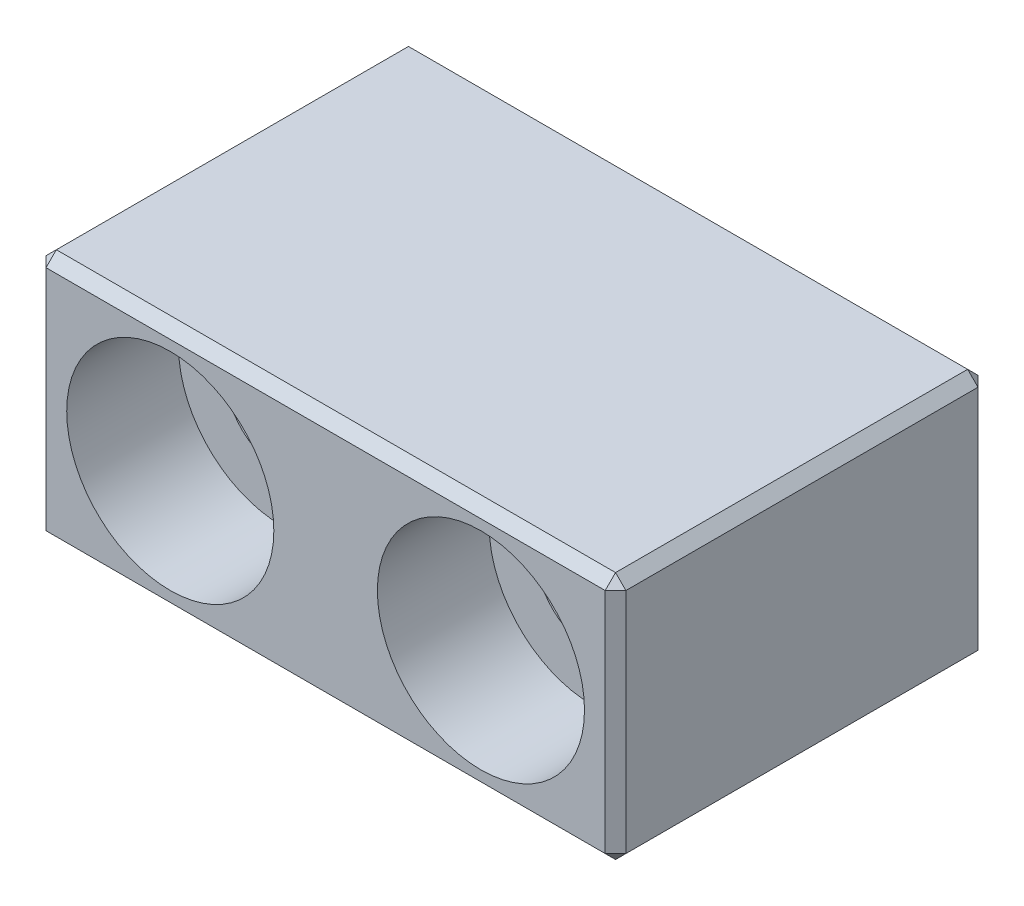
SolidWorks part; units mm, degrees
material "Al6061"
ref_plane "Front" through (0, 0, 0) normal (0, 0, 1) x (1, 0, 0)
ref_plane "Top" through (0, 0, 0) normal (0, 1, 0) x (1, 0, 0)
ref_plane "Right" through (0, 0, 0) normal (1, 0, 0) x (0, 0, -1)
sketch "草图1" plane through (0, 0, 0) normal (0, 1, 0) x (1, 0, 0)
  line L1 (-14, 9) -> (14, 9)
  line L2 (-14, 9) -> (-14, -9)
  line L3 (-14, -9) -> (14, -9)
  line L4 (14, 9) -> (14, -9)
  line L5 (-14, 9) -> (14, -9) construction
  line L6 (-14, -9) -> (14, 9) construction
  point P0 (0, 0)
  dimension "D1" = 28
  dimension "D2" = 18
extrude "凸台-拉伸1" add sketch "草图1" along normal blind 12
hole_wizard "M5 六角凹头螺钉的柱形沉头孔1" positions "草图3" profile "草图2" counterbore size "M5" standard "Iso" end condition through all
sketch "草图3" plane through (0, 0, 9) normal (0, 0, 1) x (1, 0, 0)
  line L0 (0, 0) -> (0, 12) construction
  line L1 (-14, 0) -> (14, 0) construction
  line L2 (-14, 12) -> (14, 12) construction
  line L4 (14, 6) -> (7.5, 6) construction
  line L5 (14, 12) -> (14, 0) construction
  point P0 (-7.5, 6)
  point P2 (7.5, 6)
  dimension "D1" = 15
sketch "草图2" plane through (-7.5, 6, 9) normal (1, 0, 0) x (0, -1, 0)
  line L0 (0, 0) -> (0, 18)
  line L1 (0, 18) -> (2.75, 18)
  line L3 (2.75, 18) -> (2.75, 5.4)
  line L4 (2.75, 5.4) -> (5, 5.4)
  line L5 (5, 5.4) -> (5, 0)
  line L7 (5, 0) -> (0, 0)
  line L11 (0, -6.35) -> (0, 107.95) construction
  dimension "通孔孔直径" = 5.5
  dimension "通孔孔深度" = 18
  dimension "柱形沉头孔直径" = 10
  dimension "柱形沉头孔深度" = 5.4
chamfer "倒角1" distance 0.5 angle 45 12 edges at (0, 0, -9) (0, 0, 9) (-14, 6, -9) (-14, 0, 0) (-14, 6, 9) (0, 12, 9) (-14, 12, 0) (0, 12, -9) (14, 6, 9) (14, 12, 0) (14, 6, -9) (14, 0, 0)
